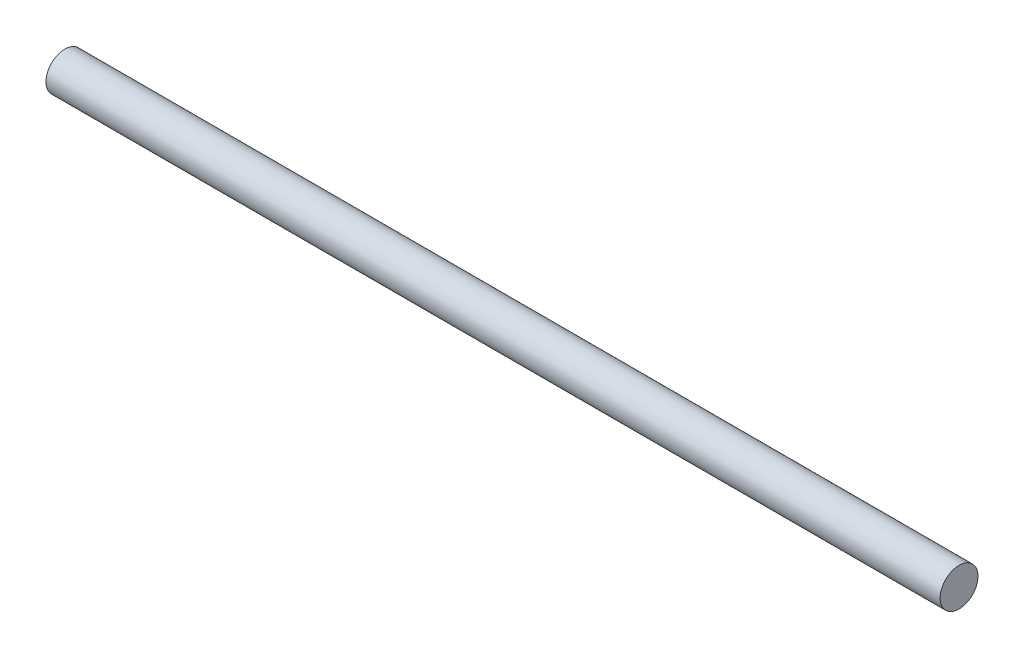
from build123d import *

# Parameters (mm, degrees)
SKETCH_1_R      = 2.5
EXTRUDE_1_DEPTH = 118


with BuildPart() as part:
    # 草图1 → 凸台-拉伸1 (new body)
    with BuildSketch(Plane(origin=(0, 0, 0), x_dir=(0, 0, -1), z_dir=(1, 0, 0))):
        Circle(SKETCH_1_R)
    extrude(amount=EXTRUDE_1_DEPTH)


solid = part.part
